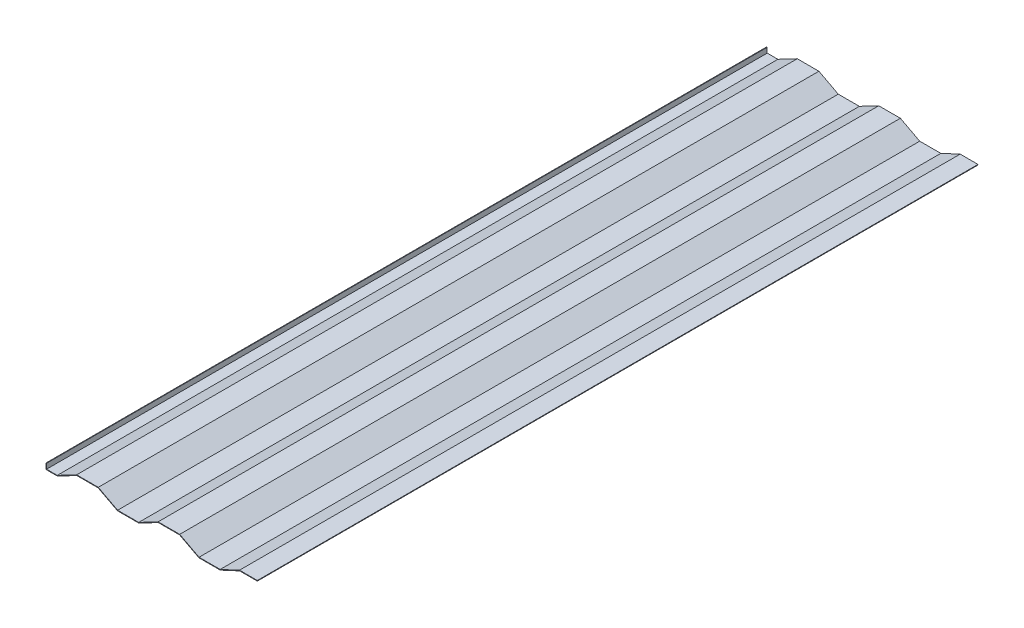
SolidWorks part; units mm, degrees
ref_plane "Front Plane" through (0, 0, 0) normal (0, 0, 1) x (1, 0, 0)
ref_plane "Top Plane" through (0, 0, 0) normal (0, 1, 0) x (1, 0, 0)
ref_plane "Right Plane" through (0, 0, 0) normal (1, 0, 0) x (0, 0, -1)
other "Configuration Table"
sketch "Sketch1" plane through (0, 0, 0) normal (0, 0, 1) x (1, 0, 0)
  line L0 (0, 20) -> (0, 0)
  line L1 (0, 0) -> (40, 0)
  line L2 (40, 0) -> (107.9731, 35.6964)
  line L3 (107.9731, 35.6964) -> (182.9731, 35.6964)
  line L4 (182.9731, 35.6964) -> (250.9462, 0)
  line L5 (250.9462, 0) -> (325.9462, 0)
  line L6 (325.9462, 0) -> (393.9193, 35.6964)
  line L7 (393.9193, 35.6964) -> (468.9193, 35.6964)
  line L8 (468.9193, 35.6964) -> (536.8923, 0)
  line L9 (536.8923, 0) -> (611.8923, 0)
  line L10 (611.8923, 0) -> (679.8654, 31.6964)
  line L11 (679.8654, 31.6964) -> (742, 31.6964)
  dimension "D1" = 40
  dimension "D2" = 107.9731
  dimension "D3" = 182.9731
  dimension "D4" = 742
  dimension "D5" = 20
  dimension "D6" = 31.6964
  dimension "D7" = 35.6964
extrude "Extrude-Thin1" add sketch "Sketch1" along normal blind 2530 thin thin type one direction reverse wall 2
